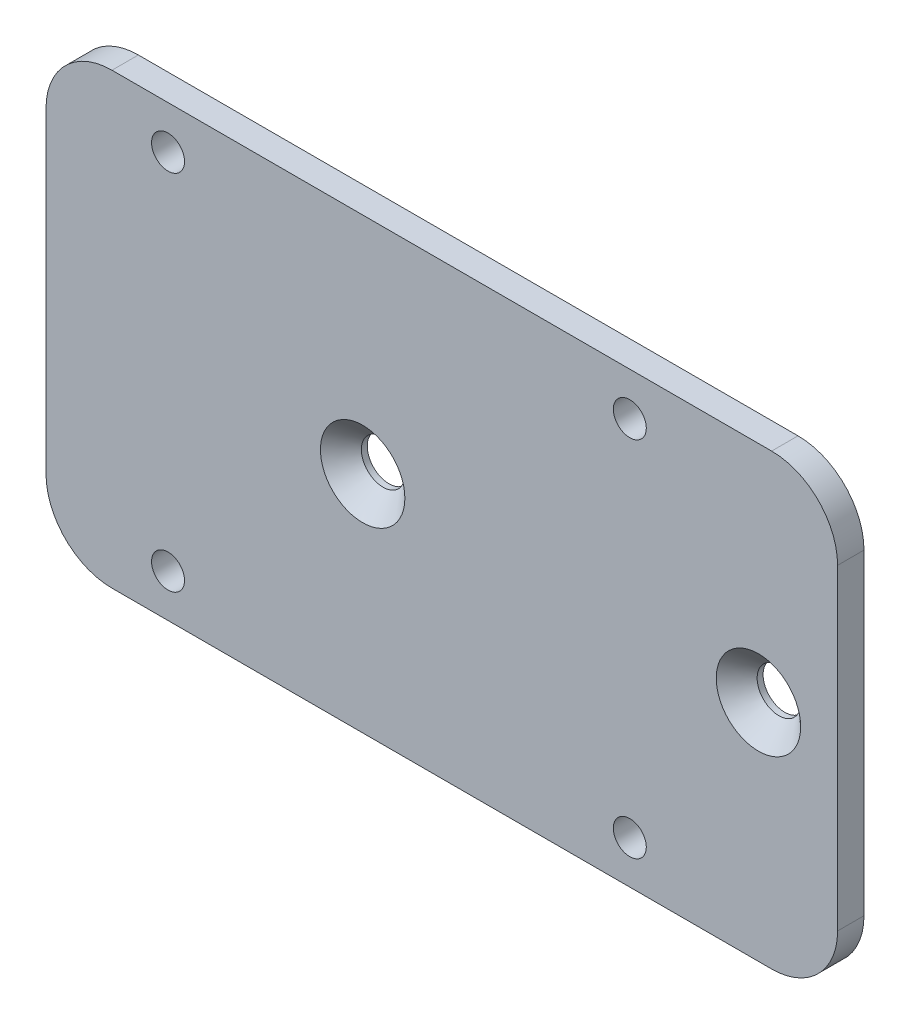
SolidWorks part; units mm, degrees
material "6061 GB/T6892-2006"
ref_plane "前视基准面" through (0, 0, 0) normal (0, 0, 1) x (1, 0, 0)
ref_plane "上视基准面" through (0, 0, 0) normal (0, 1, 0) x (1, 0, 0)
ref_plane "右视基准面" through (0, 0, 0) normal (1, 0, 0) x (0, 0, -1)
sketch "草图1" plane through (0, 0, 0) normal (0, 0, 1) x (1, 0, 0)
  line L5 (-60, 34) -> (60, 34)
  line L6 (-60, 34) -> (-60, -34)
  line L7 (-60, -34) -> (60, -34)
  line L8 (60, 34) -> (60, -34)
  line L9 (-60, 34) -> (60, -34) construction
  line L10 (-60, -34) -> (60, 34) construction
  point P0 (0, 0)
  dimension "D1" = 68
  dimension "D2" = 120
extrude "凸台-拉伸1" add sketch "草图1" along normal blind 4
hole_wizard "打孔尺寸(%根据)内六角花形半沉头螺钉的类型2" positions "草图5" profile "草图6" countersink size "M6" standard "GB"
sketch "草图5" plane through (0, 0, 0) normal (0, 0, -1) x (-1, 0, 0)
  line L1 (60, 34) -> (60, -34) construction
  point P0 (-48, 0)
  point P2 (12, 0)
  dimension "D1" = 48
  dimension "D2" = 60
sketch "草图6" plane through (48, 0, 0) normal (1, 0, 0) x (0, 1, 0)
  line L0 (0, 0) -> (0, 4)
  line L1 (0, 4) -> (3.3, 4)
  line L2 (3.3, 4) -> (3.3, 3.1)
  line L3 (3.3, 3.1) -> (6.4, 0)
  line L5 (6.4, 0) -> (0, 0)
  line L6 (-3.3, 3.1) -> (-6.4, 0) construction
  line L11 (0, -6.35) -> (0, 107.95) construction
  dimension "通孔孔直径" = 6.6
  dimension "通孔孔深度" = 4
  dimension "近端锥形沉头孔直径" = 12.8
  dimension "近端锥形沉头孔角度" = 90
sketch "草图7" plane through (0, 0, 0) normal (0, 0, -1) x (-1, 0, 0)
  point P0 (41.5, 27.5)
  point P1 (-28.5, 27.5)
  point P3 (-28.5, -27.5)
  point P5 (41.5, -27.5)
hole_wizard "M6 螺纹孔1" positions "草图3" profile "草图4" tap size "M6" standard "GB" end condition through all
sketch "草图3" plane through (0, 0, 4) normal (0, 0, 1) x (1, 0, 0)
  line L3 (0, 0) -> (48.6927, 0) construction
  point P29 (-41.5, 27.5)
  point P32 (-41.5, -27.5)
  point P35 (28.5, 27.5)
  point P38 (28.5, -27.5)
sketch "草图4" plane through (28.5, -27.5, 4) normal (1, 0, 0) x (0, -1, 0)
  line L0 (0, 0) -> (0, 4)
  line L1 (0, 4) -> (2.5, 4)
  line L2 (2.5, 4) -> (2.5, 0)
  line L5 (2.5, 0) -> (0, 0)
  line L11 (0, -6.35) -> (0, 107.95) construction
  dimension "通孔螺纹孔钻头直径" = 5
  dimension "通孔螺纹孔钻头深度" = 4
cosmetic thread "孔螺蚊线3" parameters "D2"=6
cosmetic thread "孔螺蚊线4" parameters "D2"=6
cosmetic thread "孔螺蚊线5" parameters "D2"=6
cosmetic thread "孔螺蚊线6" parameters "D2"=6
fillet "圆角1" radius 10 4 edges at (60, 34, 2) (60, -34, 2) (-60, 34, 2) (-60, -34, 2)
hole_wizard "打孔尺寸(%根据)内六角花形半沉头螺钉的类型3" positions "草图8" profile "草图9" countersink size "M6" standard "GB" end condition through all
sketch "草图8" plane through (0, 0, 4) normal (0, 0, 1) x (1, 0, 0)
  line L0 (-60, 24) -> (-60, -24) construction
  point P0 (-12, 0)
  point P2 (48, 0)
  dimension "D1" = 48
  dimension "D2" = 60
sketch "草图9" plane through (-12, 0, 4) normal (1, 0, 0) x (0, -1, 0)
  line L0 (0, 0) -> (0, 4)
  line L1 (0, 4) -> (3.3, 4)
  line L2 (3.3, 4) -> (3.3, 3.1)
  line L3 (3.3, 3.1) -> (6.4, 0)
  line L5 (6.4, 0) -> (0, 0)
  line L6 (-3.3, 3.1) -> (-6.4, 0) construction
  line L11 (0, -6.35) -> (0, 107.95) construction
  dimension "通孔孔直径" = 6.6
  dimension "通孔孔深度" = 4
  dimension "近端锥形沉头孔直径" = 12.8
  dimension "近端锥形沉头孔角度" = 90
